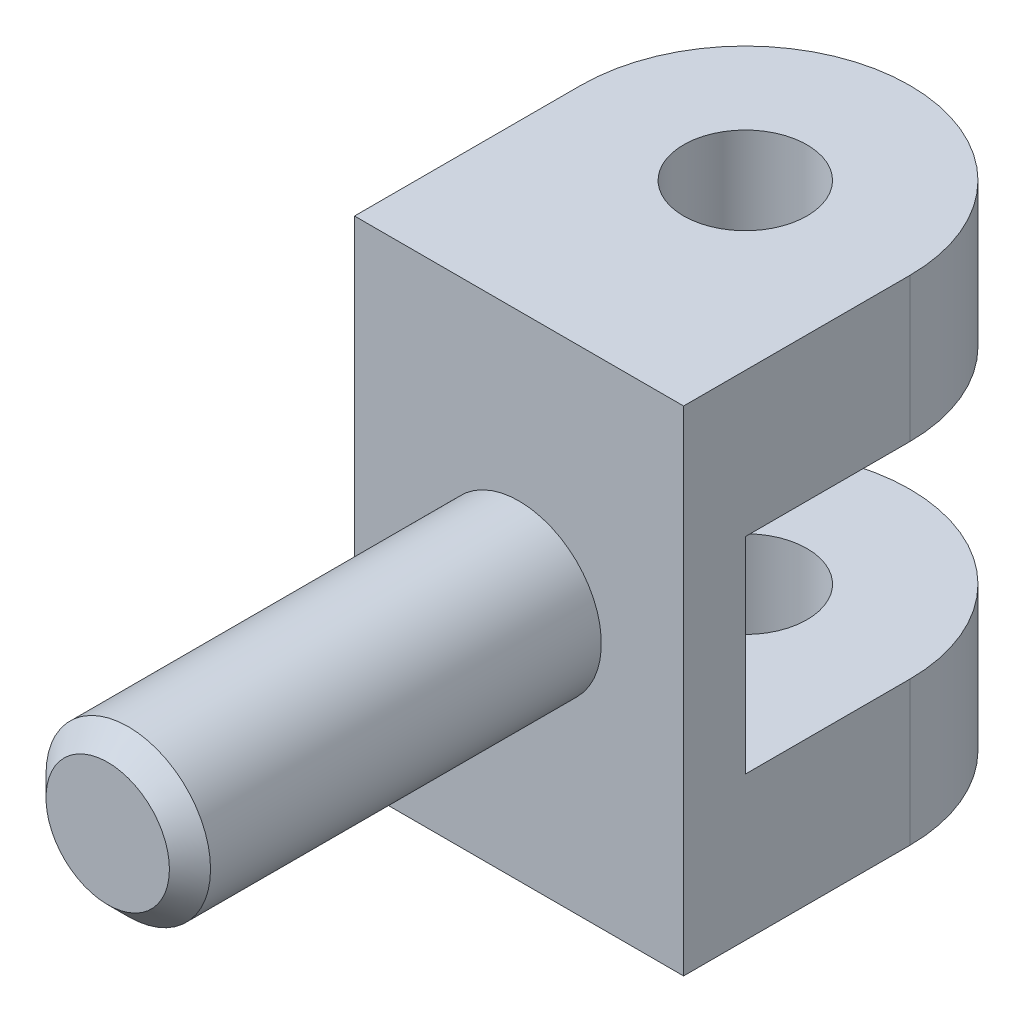
SolidWorks part; units mm, degrees
material "S45C"
ref_plane "Front" through (0, 0, 0) normal (0, 0, 1) x (1, 0, 0)
ref_plane "Top" through (0, 0, 0) normal (0, 1, 0) x (1, 0, 0)
ref_plane "Right" through (0, 0, 0) normal (1, 0, 0) x (0, 0, -1)
sketch "Sketch1" plane through (0, 0, 0) normal (0, 1, 0) x (1, 0, 0)
  line L2 (-8, 0) -> (-8, -11)
  line L3 (-8, -11) -> (8, -11)
  line L4 (8, 0) -> (8, -11)
  arc A0 (8, 0) -> (-8, 0) centre (0, 0) ccw
  dimension "D1" = 16
  dimension "D2" = 11
extrude "Boss-Extrude1" add sketch "Sketch1" along normal mid plane 24
sketch "Sketch2" plane through (0, 0, 11) normal (0, 0, 1) x (1, 0, 0)
  circle A0 centre (0, 0) radius 4
  dimension "D1" = 8
extrude "Boss-Extrude2" add sketch "Sketch2" along normal blind 20
sketch "Sketch3" plane through (8, 0, 0) normal (1, 0, 0) x (0, 0, -1)
  line L0 (8, -12) -> (8, 12) construction
  line L1 (24, 5) -> (-8, 5)
  line L2 (24, 5) -> (24, -5)
  line L3 (24, -5) -> (-8, -5)
  line L4 (-8, 5) -> (-8, -5)
  line L5 (24, 5) -> (-8, -5) construction
  line L6 (24, -5) -> (-8, 5) construction
  line L7 (-11, 12) -> (-11, -12) construction
  point P0 (8, 0)
  dimension "D1" = 10
  dimension "D2" = 3
extrude "Cut-Extrude1" cut sketch "Sketch3" against normal blind 20
sketch "Sketch4" plane through (0, -12, 0) normal (0, -1, 0) x (1, 0, 0)
  circle A0 centre (0, 0) radius 3
  dimension "D1" = 6
extrude "Cut-Extrude2" cut sketch "Sketch4" against normal blind 34
chamfer "Chamfer1" distance 1 angle 45 1 edges at (4, 0, 31)
